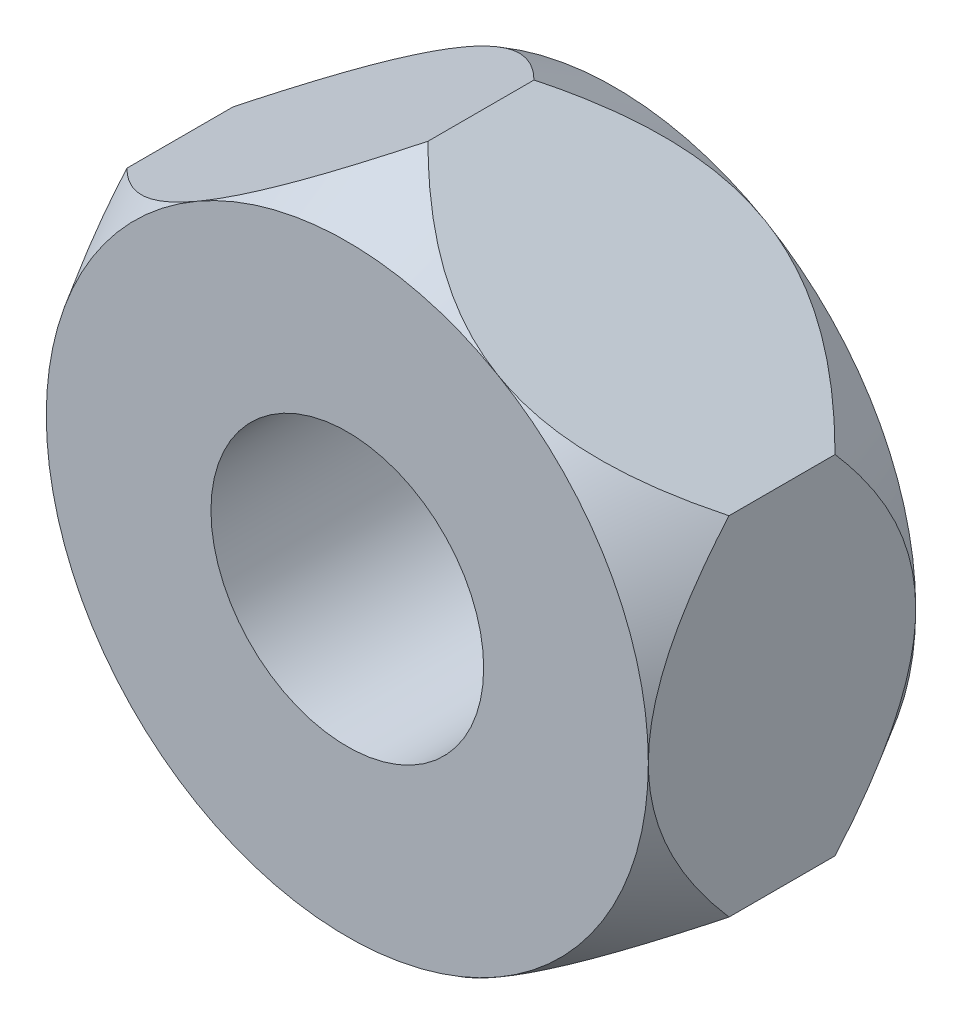
SolidWorks part; units mm, degrees
ref_plane "Front Plane" through (0, 0, 0) normal (0, 0, 1) x (1, 0, 0)
ref_plane "Top Plane" through (0, 0, 0) normal (0, 1, 0) x (1, 0, 0)
ref_plane "Right Plane" through (0, 0, 0) normal (1, 0, 0) x (0, 0, -1)
sketch "Sketch1" plane through (0, 0, 0) normal (0, 0, 1) x (1, 0, 0)
  line L1 (0, 13) -> (-11.2583, 6.5)
  line L2 (-11.2583, 6.5) -> (-11.2583, -6.5)
  line L3 (-11.2583, -6.5) -> (0, -13)
  line L4 (0, -13) -> (11.2583, -6.5)
  line L5 (11.2583, -6.5) -> (11.2583, 6.5)
  line L6 (11.2583, 6.5) -> (0, 13)
  circle A0 centre (0, 0) radius 11.2583 construction
  dimension "D1" = 26
extrude "Boss-Extrude1" add sketch "Sketch1" along normal mid plane 10
sketch "Sketch2" plane through (0, 0, 5) normal (0, 0, 1) x (1, 0, 0)
  circle A0 centre (0, 0) radius 11.2583
  dimension "D1" = 22.5167
extrude "Cut-Extrude1" cut sketch "Sketch2" against normal blind 10 draft 30 flip side to cut
mirror "Mirror1" about plane through (0, 0, 0) normal (0, 0, 1) of "Cut-Extrude1"
sketch "Sketch4" plane through (0, 0, 5) normal (0, 0, 1) x (1, 0, 0)
  point P0 (0, 0)
hole_wizard "M12 Tapped Hole3" positions "3DSketch3" profile "Sketch6" tap size "M12" standard "Gb"
sketch3d "3DSketch3"
  point P0 (0, 0, 5)
sketch "Sketch6" plane through (0, 0, 5) normal (1, 0, 0) x (0, -1, 0)
  line L0 (0, 0) -> (0, 38.75)
  line L1 (0, 38.75) -> (5.1, 38.75)
  line L2 (5.1, 38.75) -> (5.1, 0)
  line L5 (5.1, 0) -> (0, 0)
  line L10 (0, 38.75) -> (-5.1, 38.75) construction
  line L11 (0, -6.35) -> (0, 107.95) construction
  dimension "螺纹孔钻头直径" = 10.2
  dimension "螺纹孔钻头深度" = 38.75
  dimension "导头角度" = 180
cosmetic thread "CosmeticThread Hole3" parameters "D1"=10, "D2"=12
